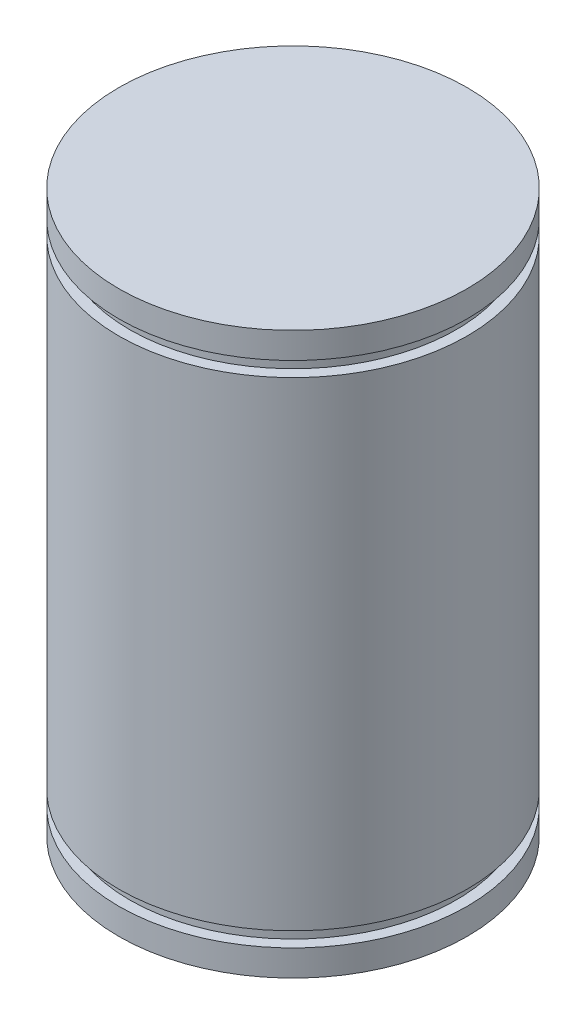
from build123d import *

# Parameters (mm, degrees)
SKETCH_1_R      = 20
EXTRUDE_1_DEPTH = 64.4
SKETCH_2_W      = 3.325902221
SKETCH_2_H      = 1.7


with BuildPart() as part:
    # 草图1 → 凸台-拉伸1 (new body)
    with BuildSketch(Plane(origin=(0, 0, 0), x_dir=(1, 0, 0), z_dir=(0, 1, 0))):
        with Locations(Location((0, 0, 0), (0, 0, 270))):
            Circle(SKETCH_1_R)
    extrude(amount=EXTRUDE_1_DEPTH)

    # 草图2 → 切除-旋转1 (revolve, cut)
    with BuildSketch(Plane.XY, mode=Mode.PRIVATE) as cut_revolve_1_sk:
        with Locations((-20.41295111, 60.55)):
            Rectangle(SKETCH_2_W, SKETCH_2_H)
    cut_revolve_1 = revolve(cut_revolve_1_sk.sketch.rotate(Axis((0, 64.4, 0), (0, -1, 0)), 270), axis=Axis((0, 64.4, 0), (0, -1, 0)), mode=Mode.SUBTRACT)

    # 镜向1: 切除-旋转1 across plane
    add(cut_revolve_1.mirror(Plane(origin=(0, 32.2, 0), x_dir=(0, 0, 1), z_dir=(0, -1, 0))), mode=Mode.SUBTRACT)


solid = part.part
